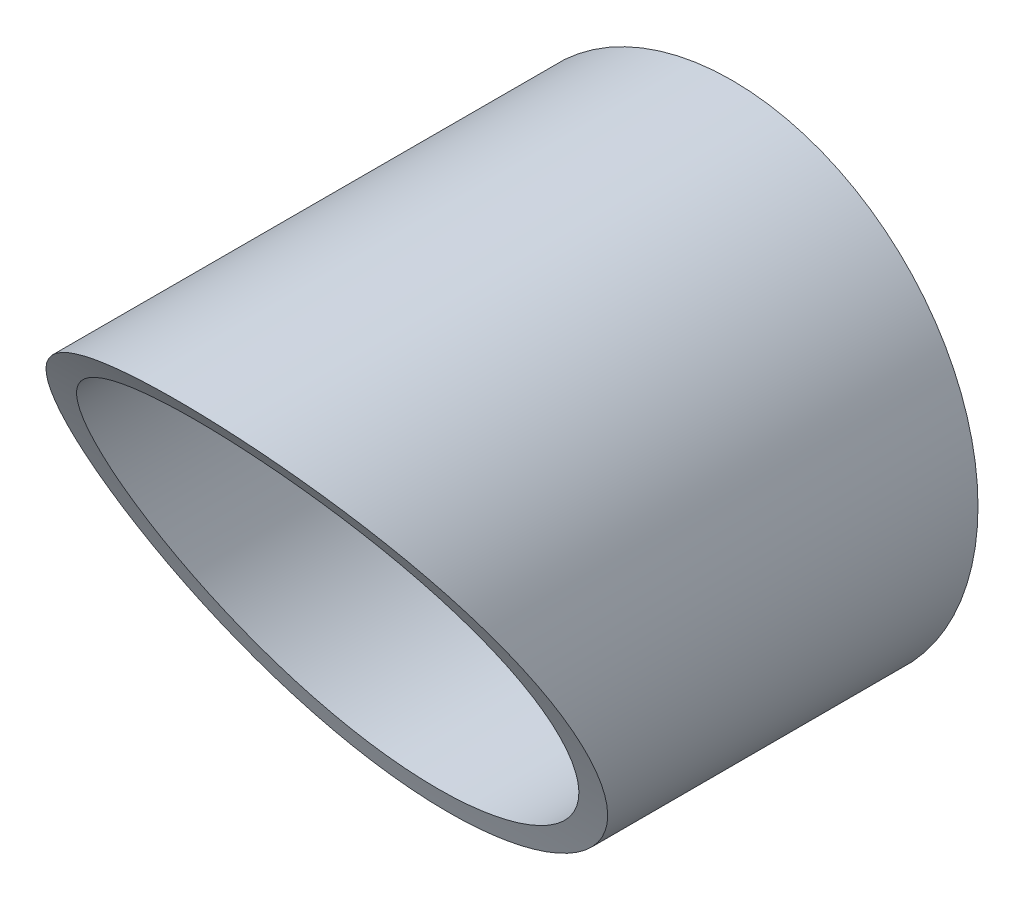
SolidWorks part; units mm, degrees
material "钢管76×4/Q235A"
ref_plane "Front Plane" through (0, 0, 0) normal (0, 0, 1) x (1, 0, 0)
ref_plane "Top Plane" through (0, 0, 0) normal (0, 1, 0) x (1, 0, 0)
ref_plane "Right Plane" through (0, 0, 0) normal (1, 0, 0) x (0, 0, -1)
sketch "Sketch1" plane through (0, 0, 0) normal (0, 0, 1) x (1, 0, 0)
  circle A0 centre (0, 0) radius 38
  circle A1 centre (0, 0) radius 34
  dimension "D1" = 76
  dimension "D2" = 4
extrude "Boss-Extrude1" add sketch "Sketch1" along normal blind 500
cosmetic thread "Cosmetic Thread1" parameters "D1"=30, "D2"=72.226
sketch "Sketch2" plane through (0, 0, 0) normal (1, 0, 0) x (0, 0, -1)
  line L0 (-500, 0) -> (0, 0) construction
  line L1 (-500, 0) -> (-395, -181.8653) construction
  line L2 (-500, 38) -> (-500, -38) construction
  circle A1 centre (-500, 0) radius 379.5 construction
  circle A3 centre (-395, -181.8653) radius 379.5
  dimension "D1" = 759
  dimension "D3" = 210
  dimension "D4" = 759
  dimension "D2" = 60
extrude "Cut-Extrude1" cut sketch "Sketch2" against normal mid plane 100
